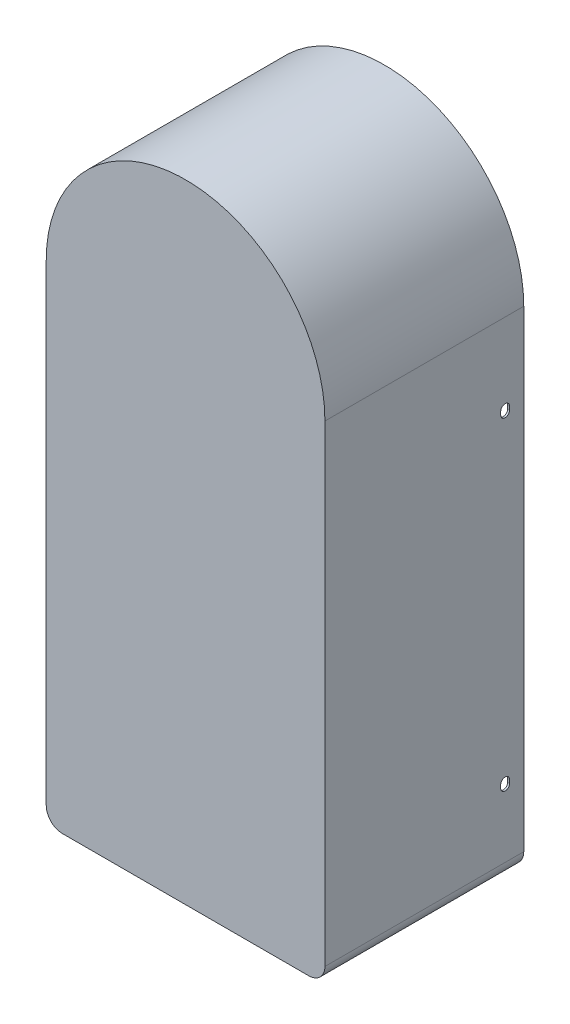
SolidWorks part; units mm, degrees
ref_plane "Front Plane" through (0, 0, 0) normal (0, 0, 1) x (1, 0, 0)
ref_plane "Top Plane" through (0, 0, 0) normal (0, 1, 0) x (1, 0, 0)
ref_plane "Right Plane" through (0, 0, 0) normal (1, 0, 0) x (0, 0, -1)
sketch "Sketch1" plane through (0, 0, 0) normal (0, 0, 1) x (1, 0, 0)
  line L0 (-86.2, -151.7) -> (-86.2, 150.5)
  line L1 (75, -150.5) -> (-75, -150.5)
  line L2 (85, -140.5) -> (85, 150.5)
  line L4 (-85, -140.5) -> (-85, 150.5)
  line L5 (85, -150.5) -> (-85, 150.5) construction
  line L6 (85, 150.5) -> (-85, -150.5) construction
  line L7 (86.2, -151.7) -> (-86.2, -151.7)
  line L8 (86.2, -151.7) -> (86.2, 150.5)
  line L9 (85, -150.5) -> (-85, -150.5) construction
  line L10 (85, -150.5) -> (85, 150.5) construction
  line L11 (-85, -150.5) -> (-85, 150.5) construction
  arc A0 (85, 150.5) -> (-85, 150.5) centre (0, 150.5) ccw
  arc A1 (86.2, 150.5) -> (-86.2, 150.5) centre (0, 150.5) ccw
  arc A2 (75, -150.5) -> (85, -140.5) centre (75, -140.5) ccw
  arc A3 (-85, -140.5) -> (-75, -150.5) centre (-75, -140.5) ccw
  point P0 (0, 0)
  dimension "D3" = 1.2
  dimension "D4" = 10
  dimension "D1" = 170
  dimension "D2" = 301
extrude "Boss-Extrude1" add sketch "Sketch1" along normal blind 123
sketch "Sketch2" plane through (0, 0, 123) normal (0, 0, 1) x (1, 0, 0)
  line L3 (-86.2, 150.5) -> (-86.2, -151.7)
  line L4 (-86.2, -151.7) -> (86.2, -151.7)
  line L5 (86.2, -151.7) -> (86.2, 150.5)
  line L6 (-86.2, 150.5) -> (-86.2, -151.7)
  line L7 (-86.2, -151.7) -> (86.2, -151.7)
  line L8 (86.2, -151.7) -> (86.2, 150.5)
  arc A1 (86.2, 150.5) -> (-86.2, 150.5) centre (0, 150.5) ccw
  arc A2 (86.2, 150.5) -> (-86.2, 150.5) centre (0, 150.5) ccw
  dimension "D1" = 0
extrude "Boss-Extrude2" add sketch "Sketch2" against normal blind 1.2
fillet "Fillet1" radius 10 1 edges at (-86.2, -151.7, 61.5)
fillet "Fillet2" radius 10 1 edges at (86.2, -151.7, 61.5)
sketch "Sketch3" plane through (-86.2, 0, 0) normal (-1, 0, 0) x (0, 0, 1)
  line L0 (11.5, 99.3) -> (11.5, 101.3) construction
  line L1 (8.75, 99.3) -> (8.75, 101.3)
  line L2 (14.25, 99.3) -> (14.25, 101.3)
  line L3 (11.5, -100.7) -> (11.5, -98.7) construction
  line L4 (8.75, -100.7) -> (8.75, -98.7)
  line L5 (14.25, -100.7) -> (14.25, -98.7)
  line L6 (0, 150.5) -> (0, -141.7) construction
  line L7 (123, -151.7) -> (0, -151.7) construction
  arc A0 (8.75, 99.3) -> (14.25, 99.3) centre (11.5, 99.3) ccw
  arc A1 (14.25, 101.3) -> (8.75, 101.3) centre (11.5, 101.3) ccw
  arc A2 (8.75, -100.7) -> (14.25, -100.7) centre (11.5, -100.7) ccw
  arc A3 (14.25, -98.7) -> (8.75, -98.7) centre (11.5, -98.7) ccw
  point P2 (11.5, 100.3)
  point P8 (11.5, -99.7)
  dimension "D2" = 2.75
  dimension "D1" = 2
  dimension "D3" = 11.5
  dimension "D4" = 52
  dimension "D5" = 200
extrude "Cut-Extrude1" cut sketch "Sketch3" against normal through all
